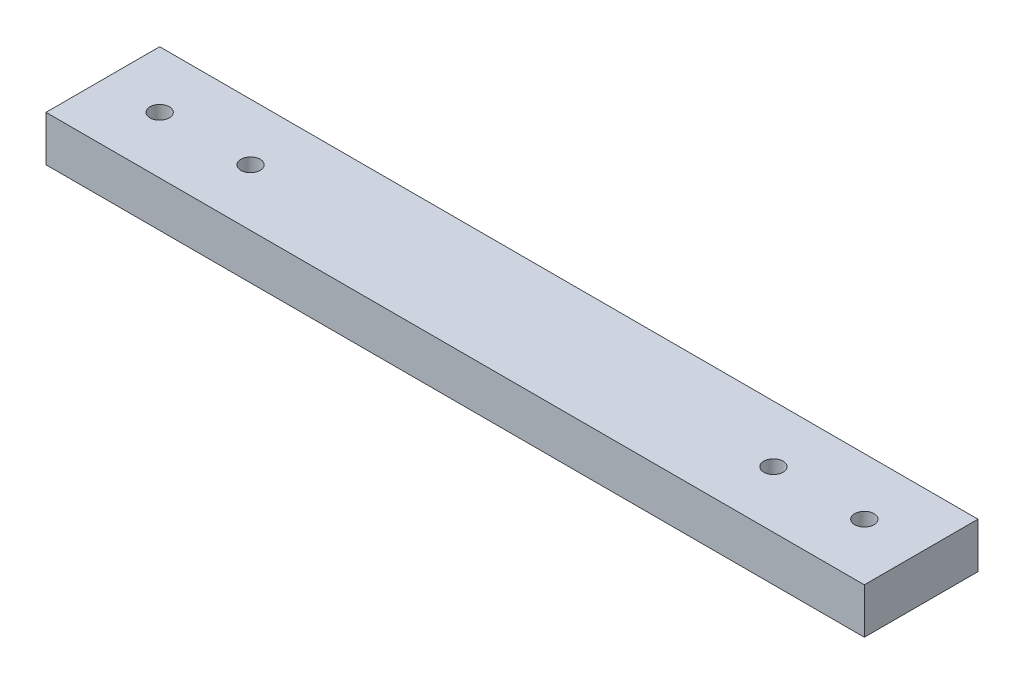
SolidWorks part; units mm, degrees
material "Q235A"
ref_plane "前视基准面" through (0, 0, 0) normal (0, 0, 1) x (1, 0, 0)
ref_plane "上视基准面" through (0, 0, 0) normal (0, 1, 0) x (1, 0, 0)
ref_plane "右视基准面" through (0, 0, 0) normal (1, 0, 0) x (0, 0, -1)
ref_plane "基准面1" through (0, 47, 0) normal (0, -1, 0) x (1, 0, 0)
sketch "草图1" plane through (0, 47, 0) normal (0, -1, 0) x (1, 0, 0)
  line L0 (360, 0) -> (0, 0)
  line L1 (0, 0) -> (0, -50)
  line L2 (0, -50) -> (360, -50)
  line L3 (360, -50) -> (360, 0)
  circle A0 centre (335, -25) radius 2.5
  circle A1 centre (65, -25) radius 2.5
  circle A2 centre (25, -25) radius 2.5
  circle A3 centre (295, -25) radius 2.5
  point P13 (0, 0)
  dimension "D1" = 5
  dimension "D2" = 25
  dimension "D3" = 65
  dimension "D4" = 295
  dimension "D5" = 335
  dimension "D6" = 360
  dimension "D7" = 25
  dimension "D8" = 50
extrude "凸台-拉伸1" add sketch "草图1" against normal blind 20
hole_wizard "M10 螺纹孔1" positions "草图2" profile "草图3" tap size "M10" standard "ISO" end condition through all
sketch "草图2" plane through (0, 47, 0) normal (0, -1, 0) x (-1, 0, 0)
  point P0 (-335, 25)
  point P3 (-295, 25)
  point P6 (-65, 25)
  point P9 (-25, 25)
sketch "草图3" plane through (335, 47, -25) normal (1, 0, 0) x (0, 0, -1)
  line L0 (0, 0) -> (0, 20)
  line L1 (0, 20) -> (4.25, 20)
  line L2 (4.25, 20) -> (4.25, 0)
  line L5 (4.25, 0) -> (0, 0)
  line L11 (0, -6.35) -> (0, 107.95) construction
  dimension "通孔螺纹孔钻头直径" = 8.5
  dimension "通孔螺纹孔钻头深度" = 20
cosmetic thread "孔螺蚊线1" parameters "D2"=10
cosmetic thread "孔螺蚊线2" parameters "D2"=10
cosmetic thread "孔螺蚊线3" parameters "D2"=10
cosmetic thread "孔螺蚊线4" parameters "D2"=10
